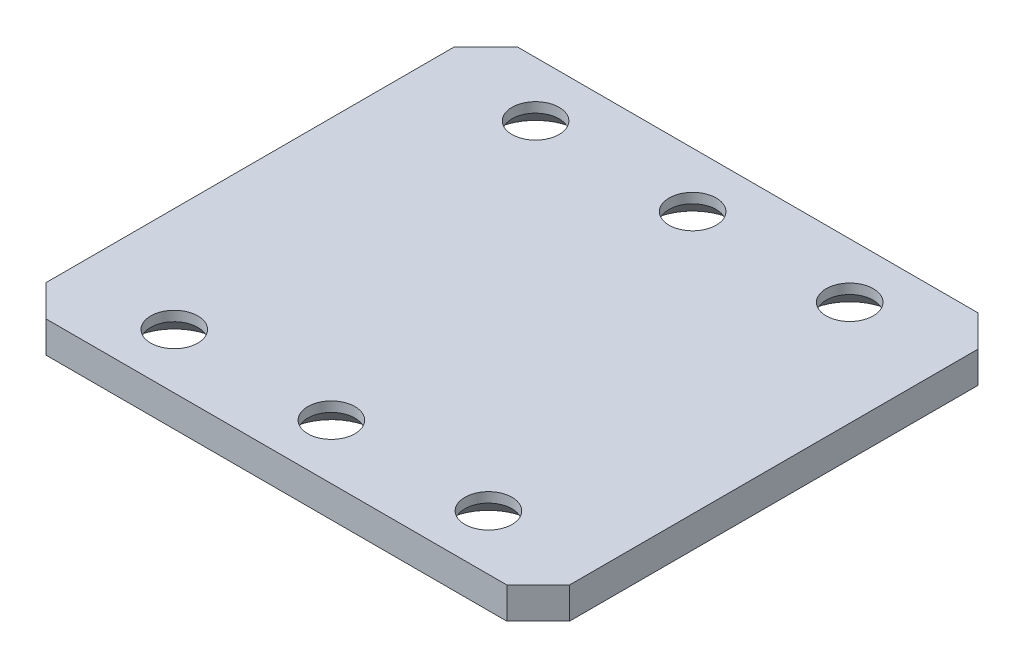
from build123d import *

# Parameters (mm, degrees)
SKETCH_1_W                = 50
SKETCH_1_H                = 45
EXTRUDE_1_DEPTH           = 3
HOLE_WIZARD_1_D           = 4.5
HOLE_WIZARD_1_DEPTH       = 12.4
HOLE_WIZARD_1_CSINK_D     = 8.6
HOLE_WIZARD_1_CSINK_ANGLE = 90
HOLE_WIZARD_1_TIP         = 1.351936393
CHAMFER_1_SIZE            = 3


with BuildPart() as part:
    # 草图1 → 凸台-拉伸1 (new body)
    with BuildSketch(Plane(origin=(0, 0, 0), x_dir=(1, 0, 0), z_dir=(0, 1, 0))):
        Rectangle(SKETCH_1_W, SKETCH_1_H)
    extrude(amount=EXTRUDE_1_DEPTH)

    # 打孔尺寸(%根据)开槽半沉头木螺钉的类型1
    with Locations(Plane(origin=(0, 0, 0), x_dir=(-1, 0, 0), z_dir=(0, -1, 0))):
        with Locations((15, 17.25), (0, 17.25), (-15, 17.25), (-15, -17.25), (0, -17.25), (15, -17.25)):
            CounterSinkHole(HOLE_WIZARD_1_D / 2, HOLE_WIZARD_1_CSINK_D / 2, depth=HOLE_WIZARD_1_DEPTH, counter_sink_angle=HOLE_WIZARD_1_CSINK_ANGLE)
            with Locations((0, 0, -(HOLE_WIZARD_1_DEPTH + HOLE_WIZARD_1_TIP / 2))):  # 118° drill point
                Cone(0, HOLE_WIZARD_1_D / 2, HOLE_WIZARD_1_TIP, mode=Mode.SUBTRACT)

    # 倒角1
    chamfer_1_edges = [part.edges().sort_by_distance(p)[0] for p in [
        (25, 1.5, 22.5),
        (-25, 1.5, 22.5),
        (-25, 1.5, -22.5),
        (25, 1.5, -22.5),
    ]]
    chamfer(chamfer_1_edges, length=CHAMFER_1_SIZE)


solid = part.part
